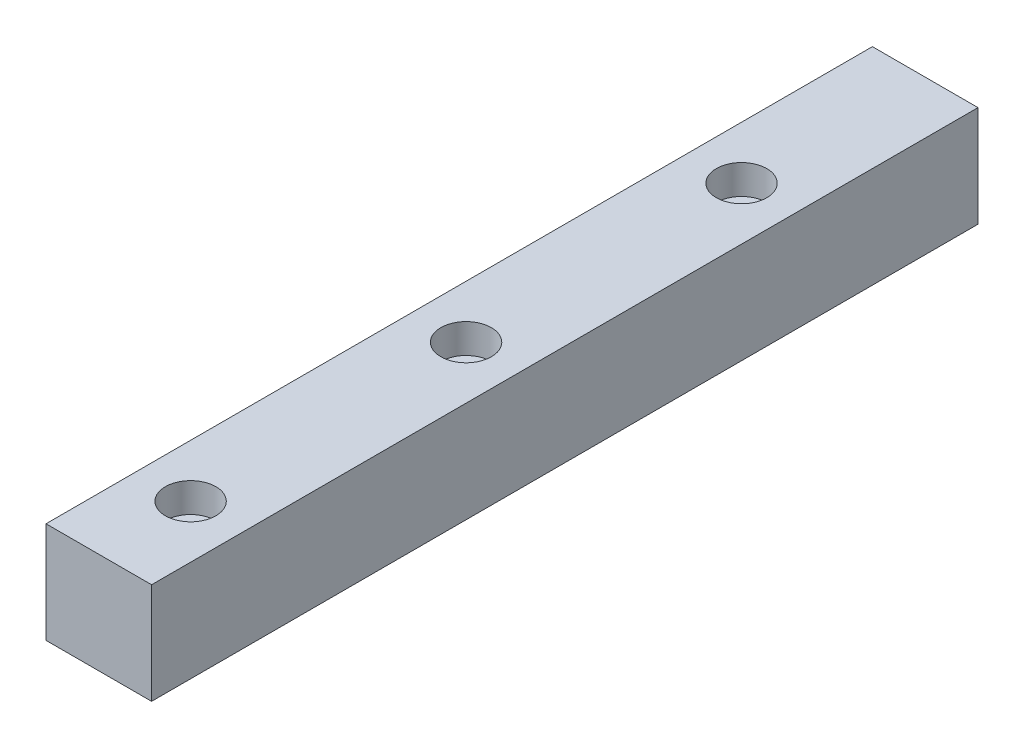
SolidWorks part; units mm, degrees
ref_plane "前视基准面" through (0, 0, 0) normal (0, 0, 1) x (1, 0, 0)
ref_plane "上视基准面" through (0, 0, 0) normal (0, 1, 0) x (1, 0, 0)
ref_plane "右视基准面" through (0, 0, 0) normal (1, 0, 0) x (0, 0, -1)
sketch "草图1" plane through (0, 0, 0) normal (0, 0, 1) x (1, 0, 0)
  line L1 (0, 0) -> (23, 0)
  line L2 (0, 0) -> (0, 22)
  line L3 (0, 22) -> (23, 22)
  line L4 (23, 0) -> (23, 22)
  dimension "D1" = 23
  dimension "D2" = 22
extrude "凸台-拉伸1" add sketch "草图1" along normal blind 180
hole_wizard "M6 六角凹头螺钉的柱形沉头孔1" positions "草图3" profile "草图4" counterbore size "M6" standard "ISO" end condition through all
sketch "草图3" plane through (0, 22, 0) normal (0, 1, 0) x (1, 0, 0)
  line L0 (11.5, -180) -> (11.5, 0) construction
  line L1 (23, -180) -> (0, -180) construction
  line L2 (23, 0) -> (0, 0) construction
  point P0 (11.5, -160)
  dimension "D1" = 20
sketch "草图4" plane through (11.5, 22, 160) normal (1, 0, 0) x (0, 0, 1)
  line L0 (0, 0) -> (0, 22)
  line L1 (0, 22) -> (3.3, 22)
  line L3 (3.3, 22) -> (3.3, 6.4)
  line L4 (3.3, 6.4) -> (5.5, 6.4)
  line L5 (5.5, 6.4) -> (5.5, 0)
  line L7 (5.5, 0) -> (0, 0)
  line L11 (0, -6.35) -> (0, 107.95) construction
  dimension "通孔孔直径" = 6.6
  dimension "通孔孔深度" = 22
  dimension "柱形沉头孔直径" = 11
  dimension "柱形沉头孔深度" = 6.4
pattern_linear "阵列(线性)1" count 4 spacing 60 along (0, 0, -1) of "M6 六角凹头螺钉的柱形沉头孔1"
